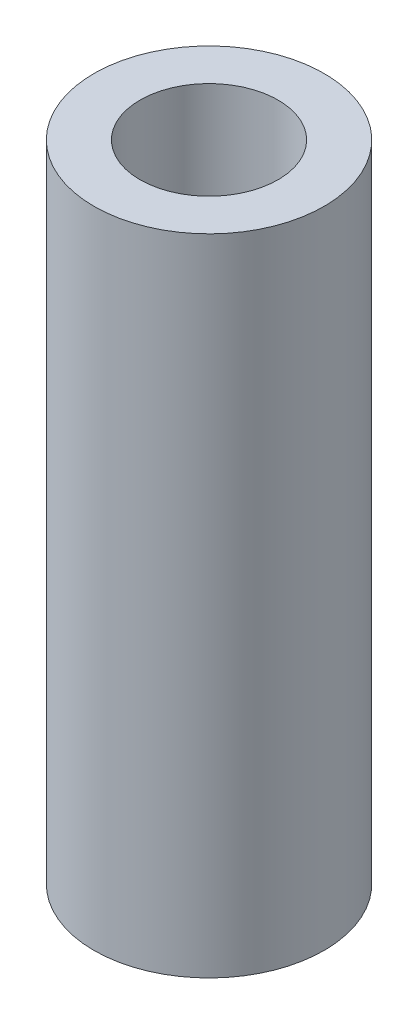
from build123d import *

# Parameters (mm, degrees)
SKETCH_1_R      = 2.5
SKETCH_1_R_2    = 1.5
EXTRUDE_1_DEPTH = 14


with BuildPart() as part:
    # 草图1 → 凸台-拉伸1 (new body)
    with BuildSketch(Plane(origin=(0, 0, 0), x_dir=(1, 0, 0), z_dir=(0, 1, 0))):
        with Locations(Location((0, 0, 0), (0, 0, 270))):
            Circle(SKETCH_1_R)
        with Locations(Location((0, 0, 0), (0, 0, 270))):
            Circle(SKETCH_1_R_2, mode=Mode.SUBTRACT)
    extrude(amount=EXTRUDE_1_DEPTH)


solid = part.part
